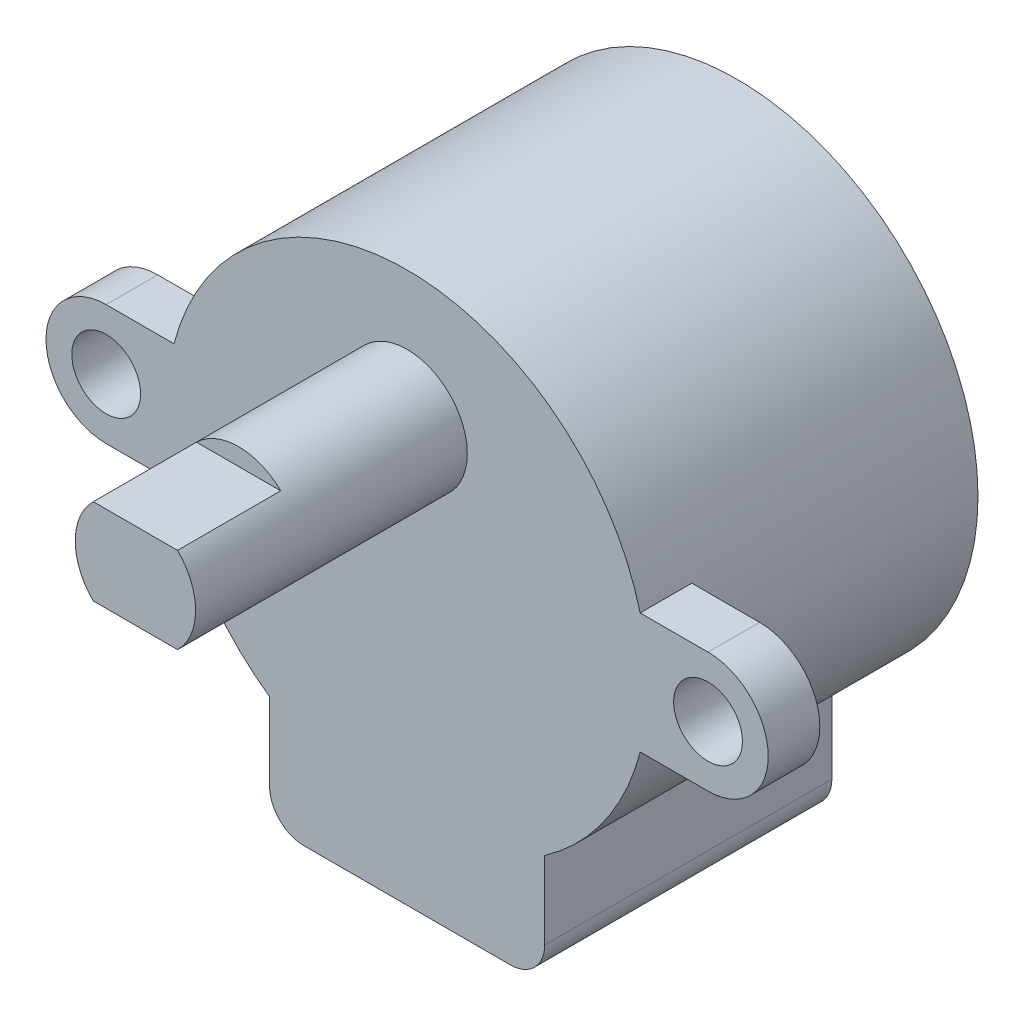
from build123d import *

# Parameters (mm, degrees)
SKETCH_1_3_R        = 2.5
BOSS_EXTRUDE1_DEPTH = 19.2
SKETCH_1_3_2_R      = 2
BOSS_EXTRUDE2_DEPTH = 3
SKETCH2_R           = 3.5
BOSS_EXTRUDE3_DEPTH = 35
CUT_EXTRUDE1_START  = -2.5
CUT_EXTRUDE1_DEPTH  = 2.5
SKETCH6_W           = 6
SKETCH6_H           = 1
CUT_EXTRUDE2_DEPTH  = 5
SCALE1_SCALE        = 0.6


with BuildPart() as part:
    # Sketch 1_3 → Boss-Extrude1 (new body)
    # profile 1 of 3: a face of its own
    with BuildSketch(Plane.XY):
        with BuildLine():
            ThreePointArc((14, 0), (0, 14), (-14, 0))
            ThreePointArc((-14, 0), (0, -14), (14, 0))
        make_face()
        with Locations((0, 6.5)):
            Circle(SKETCH_1_3_R, mode=Mode.SUBTRACT)
    # profile 2 of 3: a face of its own
    with BuildSketch(Plane.XY):
        with BuildLine():
            Line((8, -16), (8, -11.489125293))
            ThreePointArc((8, -11.489125293), (4.192388692, -13.357540082), (0, -14))
            Line((0, -14), (0, -18))
            Line((0, -18), (6, -18))
            ThreePointArc((6, -18), (7.414213562, -17.414213562), (8, -16))
        make_face()
    # profile 3 of 3: a face of its own
    with BuildSketch(Plane.XY):
        with BuildLine():
            Line((0, -18), (0, -14))
            ThreePointArc((0, -14), (-4.192388692, -13.357540082), (-8, -11.489125293))
            Line((-8, -11.489125293), (-8, -16))
            ThreePointArc((-8, -16), (-7.414213562, -17.414213562), (-6, -18))
            Line((-6, -18), (0, -18))
        make_face()
    extrude(amount=-BOSS_EXTRUDE1_DEPTH)

    # Sketch 1_3 2 → Boss-Extrude2 (add)
    # profile 1 of 2: a face of its own
    with BuildSketch(Plane.XY):
        with BuildLine():
            ThreePointArc((-14, 0), (-13.888415748, 1.764060095), (-13.555441712, 3.5))
            Line((-13.555441712, 3.5), (-17.5, 3.5))
            ThreePointArc((-17.5, 3.5), (-21, 0), (-17.5, -3.5))
            Line((-17.5, -3.5), (-13.555441712, -3.5))
            ThreePointArc((-13.555441712, -3.5), (-13.888415748, -1.764060095), (-14, 0))
        make_face()
        with Locations((-17.5, 0)):
            Circle(SKETCH_1_3_2_R, mode=Mode.SUBTRACT)
    # profile 2 of 2: a face of its own
    with BuildSketch(Plane.XY):
        with BuildLine():
            Line((13.555441712, -3.5), (17.5, -3.5))
            ThreePointArc((17.5, -3.5), (21, 0), (17.5, 3.5))
            Line((17.5, 3.5), (13.555441712, 3.5))
            ThreePointArc((13.555441712, 3.5), (13.888415748, 1.764060095), (14, 0))
            ThreePointArc((14, 0), (13.888415748, -1.764060095), (13.555441712, -3.5))
        make_face()
        with Locations((17.5, 0)):
            Circle(SKETCH_1_3_2_R, mode=Mode.SUBTRACT)
    extrude(amount=-BOSS_EXTRUDE2_DEPTH)

    # Sketch2 → Boss-Extrude3 (add)
    with BuildSketch(Plane(origin=(0, 0, -19.2), x_dir=(-1, 0, 0), z_dir=(0, 0, -1))):
        with Locations((0, 6.5)):
            Circle(SKETCH2_R)
    extrude(amount=-BOSS_EXTRUDE3_DEPTH)

    # Sketch5 → Cut-Extrude1 (cut)
    with BuildSketch(Plane(origin=(0, 0, -19.2), x_dir=(-1, 0, 0), z_dir=(0, 0, -1)).offset(CUT_EXTRUDE1_START)):
        with BuildLine():
            Line((-8, -11.489125293), (-8, -16))
            ThreePointArc((-8, -16), (-7.414213562, -17.414213562), (-6, -18))
            Line((-6, -18), (6, -18))
            ThreePointArc((6, -18), (7.414213562, -17.414213562), (8, -16))
            Line((8, -16), (8, -11.489125293))
            ThreePointArc((8, -11.489125293), (0, -14), (-8, -11.489125293))
        make_face()
    extrude(amount=CUT_EXTRUDE1_DEPTH, mode=Mode.SUBTRACT)

    # Sketch6 → Cut-Extrude2 (cut, symmetric)
    with BuildSketch(Plane(origin=(0, 0, 0), x_dir=(0, 0, -1), z_dir=(1, 0, 0))):
        with Locations((-12.8, 9.5)):
            Rectangle(SKETCH6_W, SKETCH6_H)
        with Locations((-12.8, 3.5)):
            Rectangle(SKETCH6_W, SKETCH6_H)
    extrude(amount=CUT_EXTRUDE2_DEPTH, both=True, mode=Mode.SUBTRACT)


with BuildPart() as part_1:
    # Scale1: scaled about (0, 0, 0)
    add(part.part.scale(SCALE1_SCALE))


solid = part_1.part
